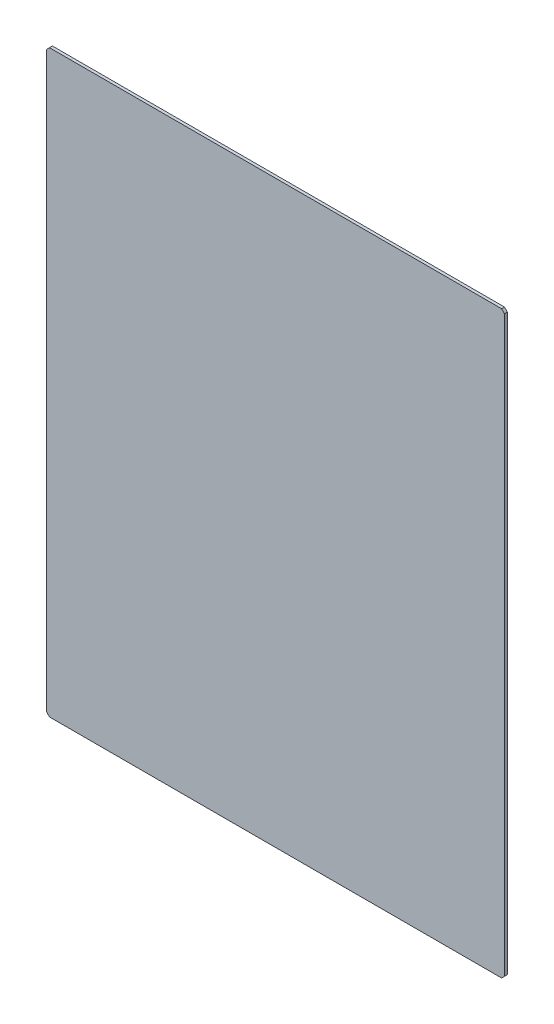
from build123d import *

# Parameters (mm, degrees)
SKETCH_1_W      = 790
SKETCH_1_H      = 1000
EXTRUDE_1_DEPTH = 5
CHAMFER_1_SIZE  = 5


with BuildPart() as part:
    # 草图1 → 拉伸1 (new body)
    with BuildSketch(Plane.XY):
        Rectangle(SKETCH_1_W, SKETCH_1_H)
    extrude(amount=EXTRUDE_1_DEPTH)

    # 倒角1
    chamfer_1_edges = [part.edges().sort_by_distance(p)[0] for p in [
        (-395, 500, 2.5),
        (395, 500, 2.5),
        (395, -500, 2.5),
        (-395, -500, 2.5),
    ]]
    chamfer(chamfer_1_edges, length=CHAMFER_1_SIZE)


solid = part.part
